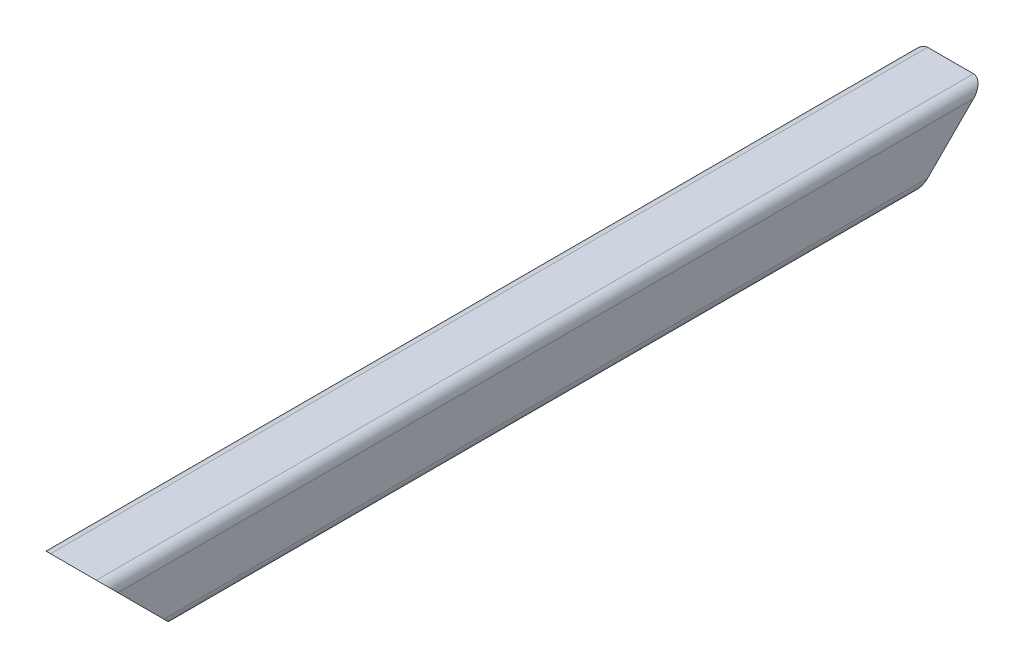
from build123d import *

# Parameters (mm, degrees)
BOSS_EXTRUDE1_DEPTH = 325
CUT_EXTRUDE1_DEPTH  = 330.772648957


with BuildPart() as part:
    # Sketch1 → Boss-Extrude1 (new, symmetric)
    with BuildSketch(Plane.XY):
        with BuildLine():
            Line((-17, -25), (17, -25))
            ThreePointArc((17, -25), (22.656854249, -22.656854249), (25, -17))
            Line((25, -17), (25, 17))
            ThreePointArc((25, 17), (22.656854249, 22.656854249), (17, 25))
            Line((17, 25), (-17, 25))
            ThreePointArc((-17, 25), (-22.656854249, 22.656854249), (-25, 17))
            Line((-25, 17), (-25, -17))
            ThreePointArc((-25, -17), (-22.656854249, -22.656854249), (-17, -25))
        make_face()
        with BuildLine():
            Line((-17, 21), (17, 21))
            ThreePointArc((17, 21), (19.828427125, 19.828427125), (21, 17))
            Line((21, 17), (21, -17))
            ThreePointArc((21, -17), (19.828427125, -19.828427125), (17, -21))
            Line((17, -21), (-17, -21))
            ThreePointArc((-17, -21), (-19.828427125, -19.828427125), (-21, -17))
            Line((-21, -17), (-21, 17))
            ThreePointArc((-21, 17), (-19.828427125, 19.828427125), (-17, 21))
        make_face(mode=Mode.SUBTRACT)
    extrude(amount=BOSS_EXTRUDE1_DEPTH, both=True)

    # Sketch2 → Cut-Extrude1 (cut, through all)
    with BuildSketch(Plane.ZY.offset(25)):
        Polygon((-325, 25), (-275, -25), (-325, -25), align=None)
    cut_extrude1 = extrude(amount=-CUT_EXTRUDE1_DEPTH, mode=Mode.SUBTRACT)

    # Mirror1: Cut-Extrude1 across plane
    add(cut_extrude1.mirror(Plane.XY), mode=Mode.SUBTRACT)


solid = part.part
